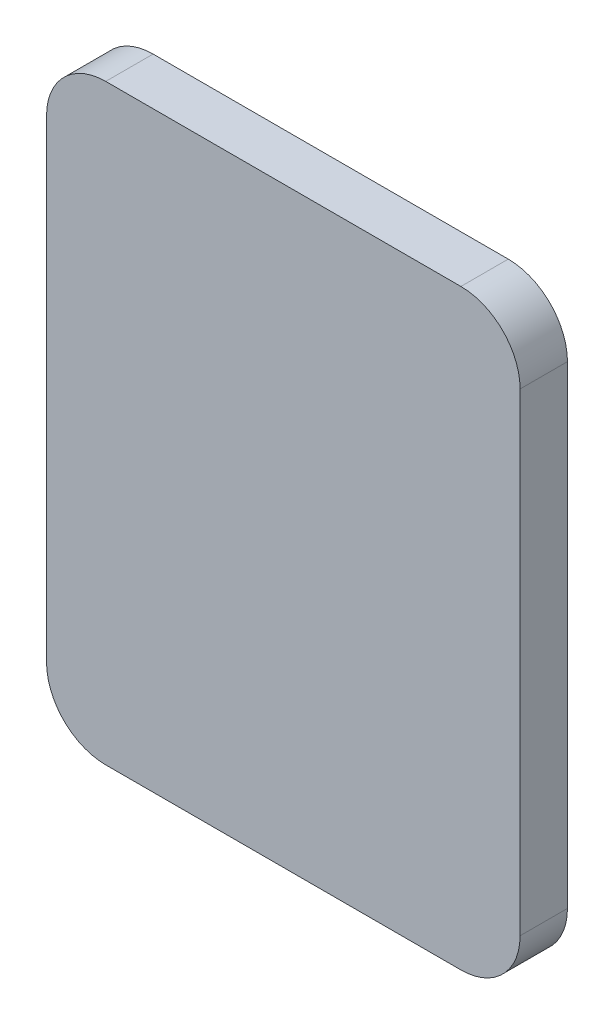
from build123d import *

# Parameters (mm, degrees)
BOSS_EXTRUDE1_DEPTH = 8


with BuildPart() as part:
    # Sketch1 → Boss-Extrude1 (new body)
    with BuildSketch(Plane.XY):
        with BuildLine():
            Line((10, 0), (70, 0))
            ThreePointArc((70, 0), (77.071067812, 2.928932188), (80, 10))
            Line((80, 10), (80, 90))
            ThreePointArc((80, 90), (77.071067812, 97.071067812), (70, 100))
            Line((70, 100), (10, 100))
            ThreePointArc((10, 100), (2.928932188, 97.071067812), (0, 90))
            Line((0, 90), (0, 10))
            ThreePointArc((0, 10), (2.928932188, 2.928932188), (10, 0))
        make_face()
    extrude(amount=BOSS_EXTRUDE1_DEPTH)


solid = part.part
